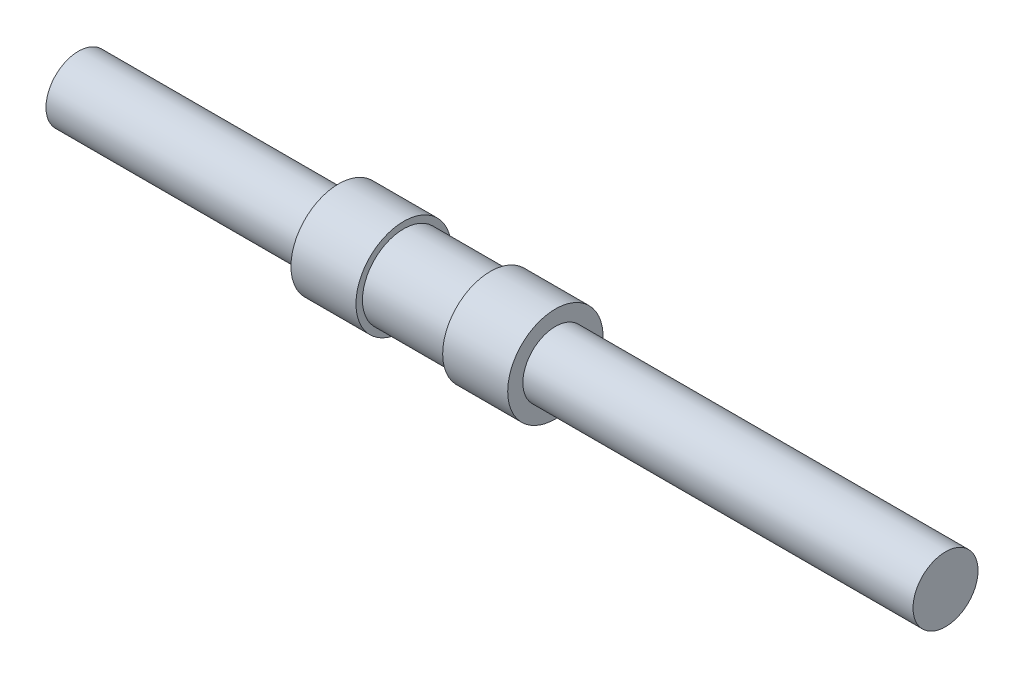
from build123d import *

# Parameters (mm, degrees)
SKETCH_2_R                = 13.5
CUT_EXTRUDE_M28_1_0_DEPTH = 300


with BuildPart() as part:
    # 草图1 → 旋转1 (revolve)
    with BuildSketch(Plane.XY, mode=Mode.PRIVATE) as revolve_1_sk:
        Polygon((0, 0), (0, 15), (120, 15), (120, 22), (150, 22), (150, 19), (190, 19), (190, 22), (220, 22), (220, 15), (400, 15), (400, 0), align=None)
    revolve(revolve_1_sk.sketch.rotate(Axis((0, 0, 0), (1, 0, 0)), 90), axis=Axis((0, 0, 0), (1, 0, 0)))

    # 草图2 → 螺纹孔M28*1.0 (cut)
    with BuildSketch(Plane.ZY):
        Circle(SKETCH_2_R)
    extrude(amount=-CUT_EXTRUDE_M28_1_0_DEPTH, mode=Mode.SUBTRACT)


solid = part.part
